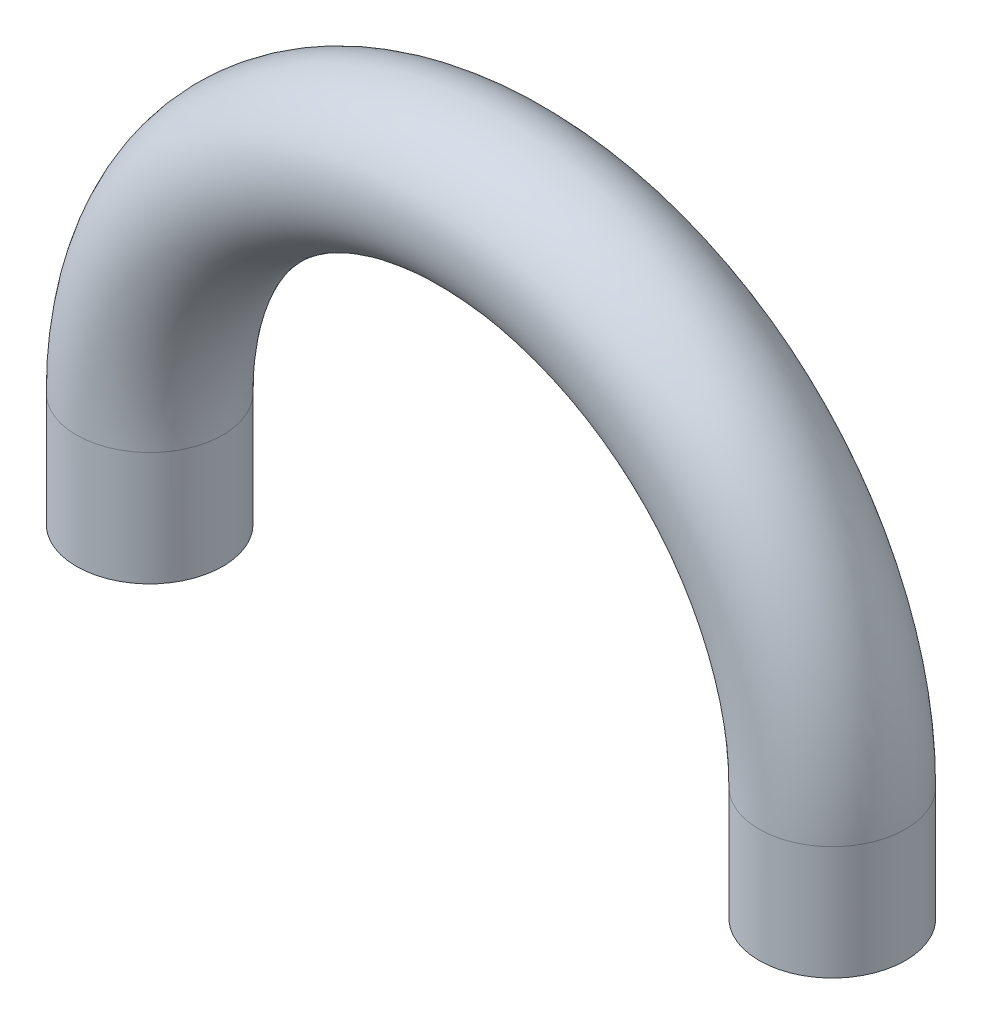
SolidWorks part; units mm, degrees
material "SS400B"
ref_plane "Front Plane" through (0, 0, 0) normal (0, 0, 1) x (1, 0, 0)
ref_plane "Top Plane" through (0, 0, 0) normal (0, 1, 0) x (1, 0, 0)
ref_plane "Right Plane" through (0, 0, 0) normal (1, 0, 0) x (0, 0, -1)
sketch "Sketch1" plane through (0, 0, 0) normal (0, 0, 1) x (1, 0, 0)
  line L0 (-21, 0) -> (21, 0) construction
  line L1 (0, 0) -> (0, 21) construction
  line L2 (-21, 0) -> (-21, -7)
  line L3 (21, 0) -> (21, -7)
  arc A0 (21, 0) -> (-21, 0) centre (0, 0) ccw
  dimension "D1" = 21
  dimension "D2" = 28
ref_plane "Plane1" through (0, -7, 0) normal (0, 1, 0) x (1, 0, 0)
sketch "Sketch4" plane through (0, -7, 0) normal (0, 1, 0) x (1, 0, 0)
  line L0 (-21, 0) -> (21, 0) construction
  line L1 (-21, 0) -> (21, 0) construction
  circle A0 centre (21, 0) radius 4.5
  dimension "D1" = 9
sweep "Sweep1" add profiles "Sketch4" path "Sketch1"
